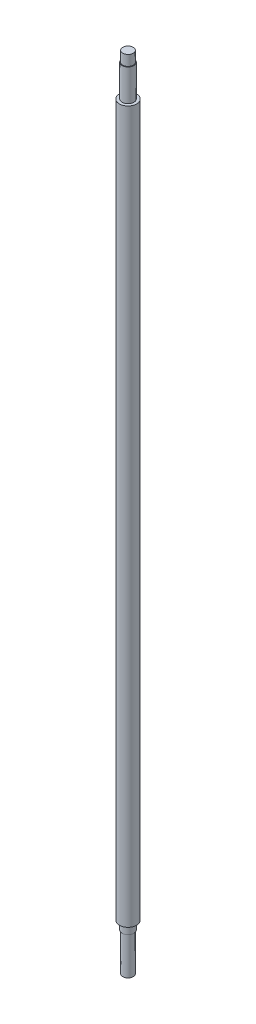
SolidWorks part; units mm, degrees
material "45"
ref_plane "Front Plane" through (0, 0, 0) normal (0, 0, 1) x (1, 0, 0)
ref_plane "Top Plane" through (0, 0, 0) normal (0, 1, 0) x (1, 0, 0)
ref_plane "Right Plane" through (0, 0, 0) normal (1, 0, 0) x (0, 0, -1)
sketch "Sketch2" plane through (0, 0, 0) normal (0, 0, 1) x (1, 0, 0)
  line L0 (0, 0) -> (0, 73.2041) construction
  line L1 (0, 0) -> (7.5, 0)
  line L2 (7.5, 0) -> (7.5, -15)
  line L3 (7.5, -15) -> (8.5, -15)
  line L4 (8.5, -15) -> (8.5, -61)
  line L5 (8.5, -61) -> (12.5, -61)
  line L6 (12.5, -61) -> (12.5, -1090)
  line L7 (12.5, -1090) -> (8.5, -1090)
  line L8 (8.5, -1090) -> (8.5, -1102)
  line L9 (8.5, -1102) -> (7.5, -1102)
  line L10 (7.5, -1102) -> (7.5, -1157)
  line L11 (7.5, -1157) -> (0, -1157)
  line L12 (0, -1157) -> (0, 0)
  dimension "D1" = 15
  dimension "D2" = 17
  dimension "D3" = 25
  dimension "D4" = 15
  dimension "D5" = 61
  dimension "D6" = 1075
  dimension "D7" = 55
  dimension "D8" = 12
revolve "Revolve1" add sketch "Sketch2" angle 360 about L0
